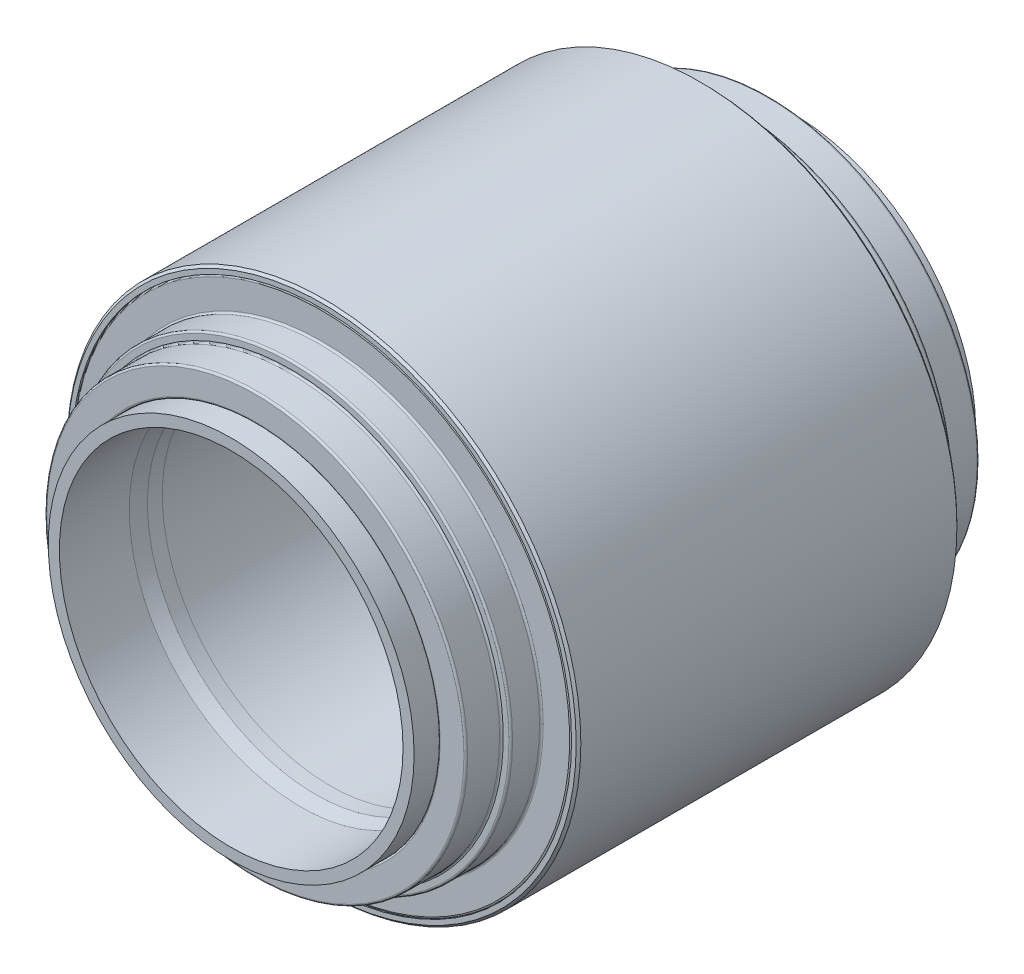
from build123d import *

# Parameters (mm, degrees)
SKETCH2_W          = 30
SKETCH2_H          = 5
SKETCH5_W          = 15.31
SKETCH5_H          = 10.31
SKETCH11_W         = 15.31
SKETCH11_H         = 10.31
FILLET1_R          = 0.8
FILLET2_R          = 0.8
CHAMFER1_SIZE      = 1
CIRPATTERN5_COUNT  = 26
CIRPATTERN7_COUNT  = 26
SKETCH14_R         = 3
CUT_EXTRUDE1_DEPTH = 198.206032164


with BuildPart() as part:
    # Sketch2 → Revolve1 (revolve)
    with BuildSketch(Plane(origin=(0, 0, 0), x_dir=(0, 0, -1), z_dir=(1, 0, 0)), mode=Mode.PRIVATE) as revolve1_sk:
        with Locations((0, 74.725)):
            Rectangle(SKETCH2_W, SKETCH2_H)
    revolve(revolve1_sk.sketch.rotate(Axis((0, 0, 191.063546837), (0, 0, -1)), 90), axis=Axis((0, 0, 191.063546837), (0, 0, -1)))


with BuildPart() as body_2:
    # Sketch3 → Revolve2 (revolve)
    with BuildSketch(Plane(origin=(0, 0, 0), x_dir=(0, 0, -1), z_dir=(1, 0, 0)), mode=Mode.PRIVATE) as revolve2_sk:
        Polygon((-21.477738984, 76.108583945), (-70.919127613, 83.796842723), (-70.252761342, 87.225), (-77.98, 87.225), (-77.98, 72.225), (-15, 72.225), (-15, 80.225), (-20.677588758, 80.225), align=None)
    revolve(revolve2_sk.sketch.rotate(Axis((0, 0, 191.063546837), (0, 0, -1)), 90), axis=Axis((0, 0, 191.063546837), (0, 0, -1)))

    # Sketch7 → Revolve7 (revolve)
    with BuildSketch(Plane(origin=(0, 0, 0), x_dir=(0, 0, -1), z_dir=(-0.9927090359250009, 0.12053534748303266, 0)), mode=Mode.PRIVATE) as revolve7_sk:
        Polygon((-66.720546233, 105.391430581), (-18.001165371, 93.999245527), (-19.73966031, 85.055464409), (-68.819056228, 94.59553256), align=None)
    revolve7 = revolve(revolve7_sk.sketch.rotate(Axis((-11.402010066, -93.905054878, 68.820228664), (0.02299922856060027, 0.18941781384606815, -0.9816271834476639)), 353.202994044), axis=Axis((-11.402010066, -93.905054878, 68.820228664), (0.02299922856060027, 0.18941781384606815, -0.9816271834476639)))

    # CirPattern5: Revolve7 ×26 about axis
    cirpattern5_axis = Axis((0, 0, 0), (0, 0, 1))
    for i in range(1, CIRPATTERN5_COUNT):
        add(revolve7.rotate(cirpattern5_axis, i * 360 / CIRPATTERN5_COUNT))


with BuildPart() as body_3:
    # Sketch4 → Revolve3 (revolve)
    with BuildSketch(Plane(origin=(0, 0, 0), x_dir=(0, 0, -1), z_dir=(1, 0, 0)), mode=Mode.PRIVATE) as revolve3_sk:
        Polygon((-77.98, 72.225), (-77.98, 77.700113365), (-87.98, 78.575), (-120.6, 78.575), (-120.6, 73.8), (-90.6, 73.8), (-84.33, 72.225), align=None)
    revolve(revolve3_sk.sketch.rotate(Axis((0, 0, 191.063546837), (0, 0, -1)), 90), axis=Axis((0, 0, 191.063546837), (0, 0, -1)))


with BuildPart() as body_4:
    # Sketch5 → Revolve4 (revolve)
    with BuildSketch(Plane(origin=(0, 0, 0), x_dir=(0, 0, -1), z_dir=(1, 0, 0)), mode=Mode.PRIVATE) as revolve4_sk:
        with Locations((-101.071, 83.73)):
            Rectangle(SKETCH5_W, SKETCH5_H)
    revolve(revolve4_sk.sketch.rotate(Axis((0, 0, 191.063546837), (0, 0, -1)), 90), axis=Axis((0, 0, 191.063546837), (0, 0, -1)))


with BuildPart() as body_5:
    # Sketch6 → Revolve5 (revolve)
    with BuildSketch(Plane(origin=(0, 0, 0), x_dir=(0, 0, -1), z_dir=(1, 0, 0)), mode=Mode.PRIVATE) as revolve5_sk:
        Polygon((-68.596, 107.331), (-68.596, 105.831), (-80.256, 105.831), (-80.256, 92.885), (-93.416, 92.885), (-93.416, 88.885), (-108.726, 88.885), (-108.726, 78.575), (-110.226, 78.575), (-110.226, 90.385), (-94.916, 90.385), (-94.916, 94.385), (-81.756, 94.385), (-81.756, 107.331), align=None)
    revolve(revolve5_sk.sketch.rotate(Axis((0, 0, 191.063546837), (0, 0, -1)), 90), axis=Axis((0, 0, 191.063546837), (0, 0, -1)))

    # Fillet1
    fillet1_edges = [body_5.edges().sort_by_distance(p)[0] for p in [
        (-78.575, 0, 110.226),
        (-90.385, 0, 110.226),
        (-90.385, 0, 94.916),
        (-94.385, 0, 94.916),
        (-94.385, 0, 81.756),
        (-107.331, 0, 81.756),
    ]]
    fillet(fillet1_edges, radius=FILLET1_R)


with BuildPart() as body_6:
    # Sketch9 → Revolve9 (revolve)
    with BuildSketch(Plane(origin=(0, 0, 0), x_dir=(0, 0, -1), z_dir=(1, 0, 0)), mode=Mode.PRIVATE) as revolve9_sk:
        Polygon((70.919127613, 83.796842723), (70.252761342, 87.225), (77.98, 87.225), (77.98, 72.225), (15, 72.225), (15, 80.225), (20.677588758, 80.225), (21.477738984, 76.108583945), align=None)
    revolve(revolve9_sk.sketch.rotate(Axis((0, 0, 191.063546837), (0, 0, -1)), 90), axis=Axis((0, 0, 191.063546837), (0, 0, -1)))

    # Sketch13 → Revolve13 (revolve)
    with BuildSketch(Plane(origin=(0, 0, 0), x_dir=(0, 0, -1), z_dir=(-0.9927090359250009, 0.12053534748303266, 0)), mode=Mode.PRIVATE) as revolve13_sk:
        Polygon((18.000782413, -93.315857585), (19.739851675, -84.434352157), (68.835859253, -93.830432782), (66.722112128, -104.62543501), align=None)
    revolve13 = revolve(revolve13_sk.sketch.rotate(Axis((10.177323977, 83.818744329, -19.739851675), (0.022657069015928375, 0.1865998448534325, -0.982174707027361)), 173.199238366), axis=Axis((10.177323977, 83.818744329, -19.739851675), (0.022657069015928375, 0.1865998448534325, -0.982174707027361)))

    # CirPattern7: Revolve13 ×26 about axis
    cirpattern7_axis = Axis((0, 0, 191.063546837), (0, 0, -1))
    for i in range(1, CIRPATTERN7_COUNT):
        add(revolve13.rotate(cirpattern7_axis, i * 360 / CIRPATTERN7_COUNT))


with BuildPart() as body_7:
    # Sketch10 → Revolve10 (revolve)
    with BuildSketch(Plane(origin=(0, 0, 0), x_dir=(0, 0, -1), z_dir=(1, 0, 0)), mode=Mode.PRIVATE) as revolve10_sk:
        Polygon((90.6, 73.8), (84.33, 72.225), (77.98, 72.225), (77.98, 77.700113365), (87.98, 78.575), (120.6, 78.575), (120.6, 73.8), align=None)
    revolve(revolve10_sk.sketch.rotate(Axis((0, 0, 191.063546837), (0, 0, -1)), 90), axis=Axis((0, 0, 191.063546837), (0, 0, -1)))

    # Sketch14 → Cut-Extrude1 (cut, through all)
    with BuildSketch(Plane(origin=(0, 0, 0), x_dir=(1, 0, 0), z_dir=(0, 1, 0))):
        with Locations((0, 120.6)):
            Circle(SKETCH14_R)
    extrude(amount=CUT_EXTRUDE1_DEPTH, mode=Mode.SUBTRACT)


with BuildPart() as body_8:
    # Sketch11 → Revolve11 (revolve)
    with BuildSketch(Plane(origin=(0, 0, 0), x_dir=(0, 0, -1), z_dir=(1, 0, 0)), mode=Mode.PRIVATE) as revolve11_sk:
        with Locations((101.071, 83.73)):
            Rectangle(SKETCH11_W, SKETCH11_H)
    revolve(revolve11_sk.sketch.rotate(Axis((0, 0, 191.063546837), (0, 0, -1)), 90), axis=Axis((0, 0, 191.063546837), (0, 0, -1)))


with BuildPart() as body_9:
    # Sketch12 → Revolve12 (revolve)
    with BuildSketch(Plane(origin=(0, 0, 0), x_dir=(0, 0, -1), z_dir=(1, 0, 0)), mode=Mode.PRIVATE) as revolve12_sk:
        Polygon((110.226, 78.575), (108.726, 78.575), (108.726, 88.885), (93.416, 88.885), (93.416, 92.885), (80.256, 92.885), (80.256, 105.831), (68.596, 105.831), (68.596, 107.331), (81.756, 107.331), (81.756, 94.385), (94.916, 94.385), (94.916, 90.385), (110.226, 90.385), align=None)
    revolve(revolve12_sk.sketch.rotate(Axis((0, 0, 0), (0, 0, 1)), 90), axis=Axis((0, 0, 0), (0, 0, 1)))

    # Fillet2
    fillet2_edges = [body_9.edges().sort_by_distance(p)[0] for p in [
        (107.331, 0, -81.756),
        (94.385, 0, -81.756),
        (94.385, 0, -94.916),
        (90.385, 0, -94.916),
        (90.385, 0, -110.226),
        (78.575, 0, -110.226),
    ]]
    fillet(fillet2_edges, radius=FILLET2_R)


with BuildPart() as body_10:
    # Sketch8 → Revolve8 (revolve)
    with BuildSketch(Plane(origin=(0, 0, 0), x_dir=(0, 0, -1), z_dir=(1, 0, 0)), mode=Mode.PRIVATE) as revolve8_sk:
        Polygon((-68.596, 107.331), (-68.596, 105.831), (-18, 94), (18, 94), (68.596, 105.831), (68.596, 107.331), (81.756, 107.331), (81.756, 110.331), (-81.756, 110.331), (-81.756, 107.331), align=None)
    revolve(revolve8_sk.sketch.rotate(Axis((0, 0, 191.063546837), (0, 0, -1)), 90), axis=Axis((0, 0, 191.063546837), (0, 0, -1)))

    # Chamfer1
    chamfer1_edges = [body_10.edges().sort_by_distance(p)[0] for p in [
        (-110.331, 0, -81.756),
        (-110.331, 0, 81.756),
    ]]
    chamfer(chamfer1_edges, length=CHAMFER1_SIZE)


solid = Compound([part.part, body_2.part, body_3.part, body_4.part, body_5.part, body_6.part, body_7.part, body_8.part, body_9.part, body_10.part])
